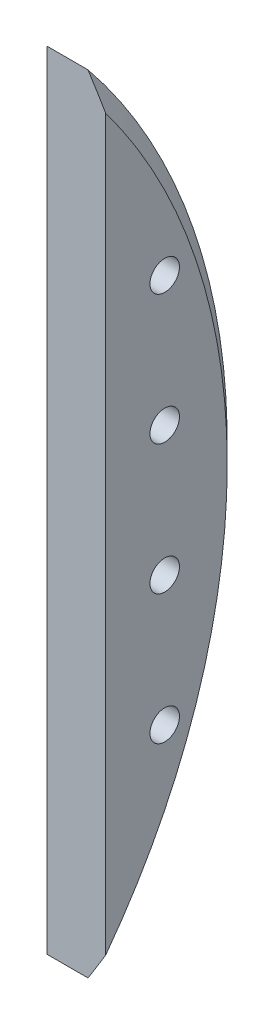
from build123d import *

# Parameters (mm, degrees)
BOSS_EXTRUDE1_DEPTH = 25
SKETCH2_R           = 12.5
CUT_EXTRUDE1_DEPTH  = 81
CHAMFER2_SIZE       = 15


with BuildPart() as part:
    # Sketch1 → Boss-Extrude1 (new, symmetric)
    with BuildSketch(Plane(origin=(0, 0, 0), x_dir=(0, 0, -1), z_dir=(1, 0, 0))):
        with BuildLine():
            Line((412, 333.400659867), (412, -333.400659867))
            ThreePointArc((412, -333.400659867), (530, 0), (412, 333.400659867))
        make_face()
    extrude(amount=BOSS_EXTRUDE1_DEPTH, both=True)

    # Sketch2 → Cut-Extrude1 (cut)
    with BuildSketch(Plane(origin=(25, 0, 0), x_dir=(0, 0, -1), z_dir=(1, 0, 0))):
        with Locations((462, 55)):
            Circle(SKETCH2_R)
        with Locations((462, -55)):
            Circle(SKETCH2_R)
        with Locations((462, 165)):
            Circle(SKETCH2_R)
        with Locations((462, -165)):
            Circle(SKETCH2_R)
    extrude(amount=-CUT_EXTRUDE1_DEPTH, mode=Mode.SUBTRACT)

    # Chamfer2
    chamfer2_edges = [part.edges().sort_by_distance(p)[0] for p in [
        (25, 0, -530),
    ]]
    chamfer(chamfer2_edges, length=CHAMFER2_SIZE)


solid = part.part
